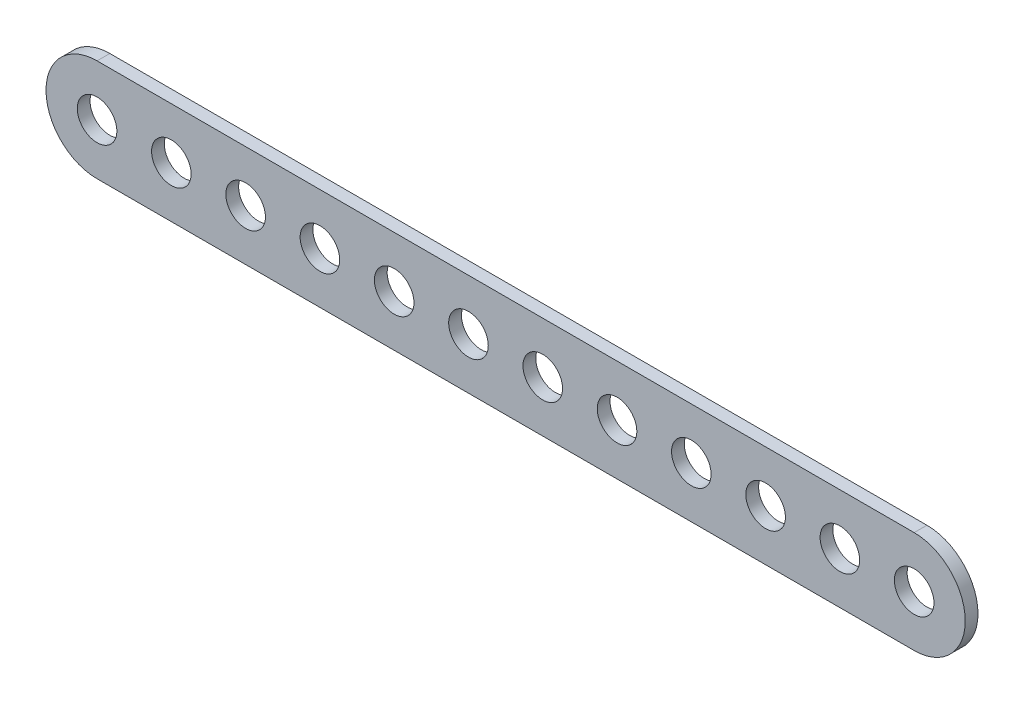
from build123d import *

# Parameters (mm, degrees)
SKETCH_1_R      = 1.55
EXTRUDE_1_DEPTH = 1


with BuildPart() as part:
    # 草图1 → 凸台-拉伸1 (new body)
    with BuildSketch(Plane.XY):
        with BuildLine():
            Line((0, 4), (64, 4))
            ThreePointArc((64, 4), (68, 0), (64, -4))
            Line((64, -4), (0, -4))
            ThreePointArc((0, -4), (-4, 0), (0, 4))
        make_face()
        Circle(SKETCH_1_R, mode=Mode.SUBTRACT)
        with Locations((5.818181818, 0)):
            Circle(SKETCH_1_R, mode=Mode.SUBTRACT)
        with Locations((11.636363636, 0)):
            Circle(SKETCH_1_R, mode=Mode.SUBTRACT)
        with Locations((17.454545455, 0)):
            Circle(SKETCH_1_R, mode=Mode.SUBTRACT)
        with Locations((23.272727273, 0)):
            Circle(SKETCH_1_R, mode=Mode.SUBTRACT)
        with Locations((29.090909091, 0)):
            Circle(SKETCH_1_R, mode=Mode.SUBTRACT)
        with Locations((34.909090909, 0)):
            Circle(SKETCH_1_R, mode=Mode.SUBTRACT)
        with Locations((40.727272727, 0)):
            Circle(SKETCH_1_R, mode=Mode.SUBTRACT)
        with Locations((46.545454545, 0)):
            Circle(SKETCH_1_R, mode=Mode.SUBTRACT)
        with Locations((52.363636364, 0)):
            Circle(SKETCH_1_R, mode=Mode.SUBTRACT)
        with Locations((58.181818182, 0)):
            Circle(SKETCH_1_R, mode=Mode.SUBTRACT)
        with Locations((64, 0)):
            Circle(SKETCH_1_R, mode=Mode.SUBTRACT)
    extrude(amount=EXTRUDE_1_DEPTH)


solid = part.part
